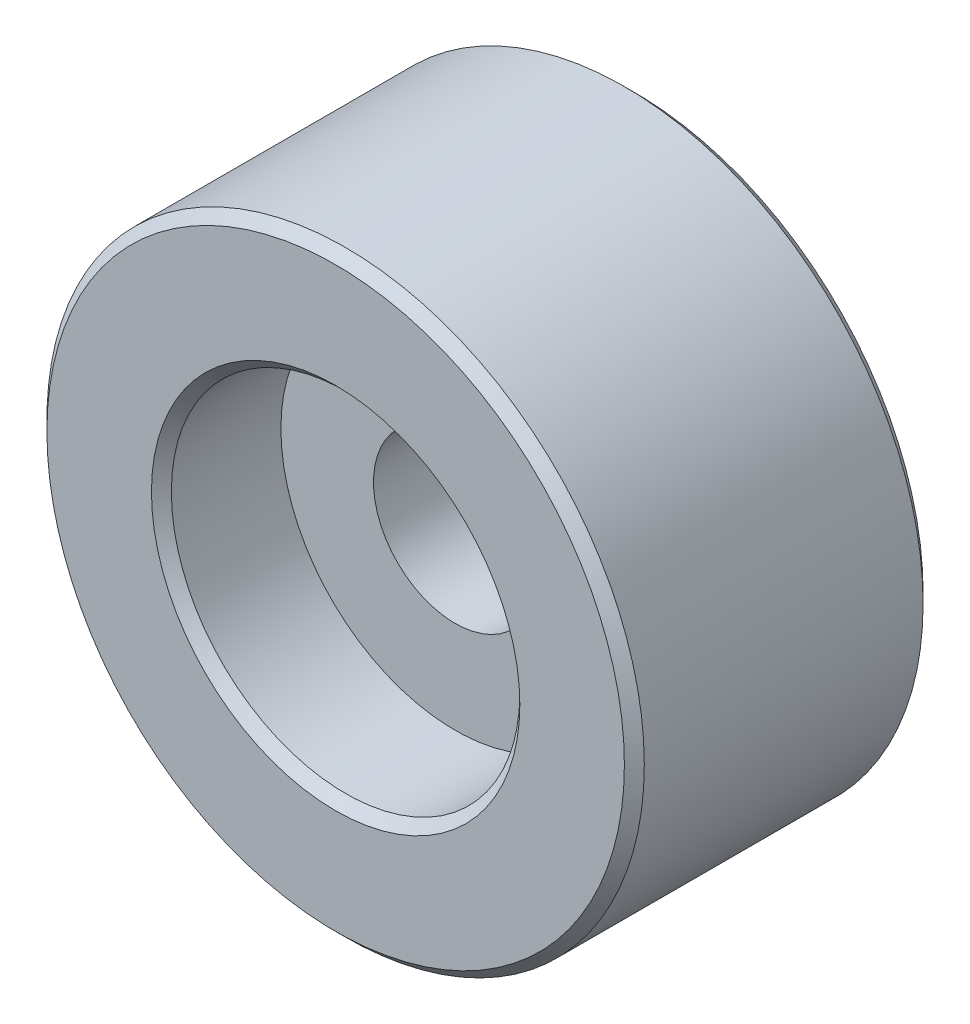
SolidWorks part; units mm, degrees
material "P20"
ref_plane "Front/Back" through (0, 0, 0) normal (0, 0, 1) x (1, 0, 0)
ref_plane "Top/Bottom" through (0, 0, 0) normal (0, 1, 0) x (1, 0, 0)
ref_plane "Right/Left" through (0, 0, 0) normal (1, 0, 0) x (0, 0, -1)
sketch "Sketch1" plane through (0, 0, 0) normal (0, 0, 1) x (1, 0, 0)
  circle A0 centre (0, 0) radius 15
  dimension "D1" = 30
extrude "Boss-Extrude1" add sketch "Sketch1" along normal blind 15
sketch "Sketch6" plane through (0, 0, 0) normal (0, 0, -1) x (-1, 0, 0)
  circle A0 centre (0, 0) radius 4.1
  dimension "D1" = 8.2
extrude "Cut-Extrude3" cut sketch "Sketch6" against normal blind 50
sketch "Sketch8" plane through (0, 0, 15) normal (0, 0, 1) x (1, 0, 0)
  circle A0 centre (0, 0) radius 8.75
  dimension "D1" = 17.5
extrude "Cut-Extrude5" cut sketch "Sketch8" against normal blind 6
chamfer "Chamfer2" distance 0.5 angle 45 1 edges at (8.75, 0, 15)
chamfer "Chamfer3" distance 0.5 angle 45 3 edges at (-4.1, 0, 0) (15, 0, 15) (15, 0, 0)
